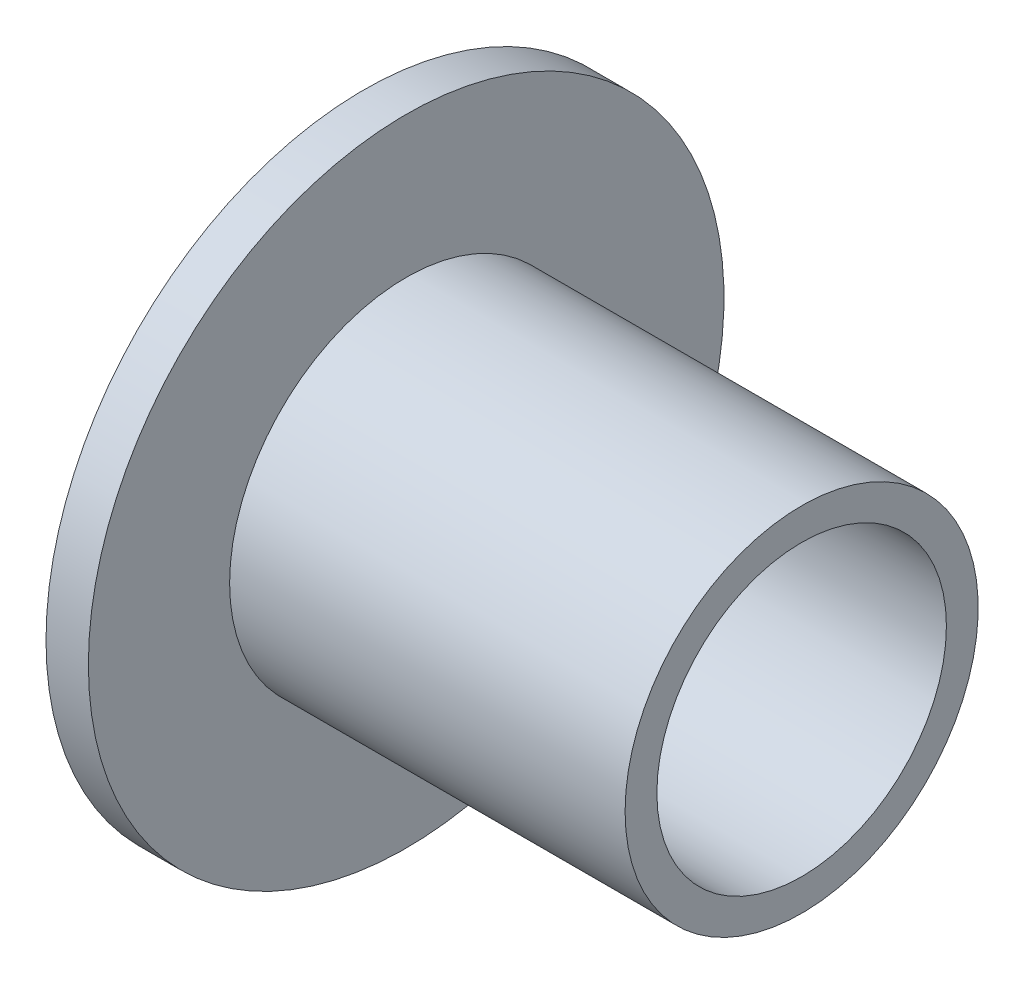
SolidWorks part; units mm, degrees
material "尼龙 101"
ref_plane "前视基准面" through (0, 0, 0) normal (0, 0, 1) x (1, 0, 0)
ref_plane "上视基准面" through (0, 0, 0) normal (0, 1, 0) x (1, 0, 0)
ref_plane "右视基准面" through (0, 0, 0) normal (1, 0, 0) x (0, 0, -1)
sketch "草图1" plane through (0, 0, 0) normal (0, 0, 1) x (1, 0, 0)
  line L0 (0, 0) -> (41.9789, 0) construction
  line L1 (0, 4.1) -> (0, 9)
  line L2 (0, 9) -> (1.2, 9)
  line L3 (1.2, 9) -> (1.2, 5)
  line L4 (1.2, 5) -> (12.4, 5)
  line L5 (12.4, 5) -> (12.4, 4.1)
  line L6 (12.4, 4.1) -> (0, 4.1)
  line L7 (0, 0) -> (0, 22.0485) construction
  dimension "D1" = 18
  dimension "D2" = 1.2
  dimension "D3" = 10
  dimension "D4" = 8.2
  dimension "D5" = 12.4
revolve "旋转1" add sketch "草图1" angle 360 about L0
